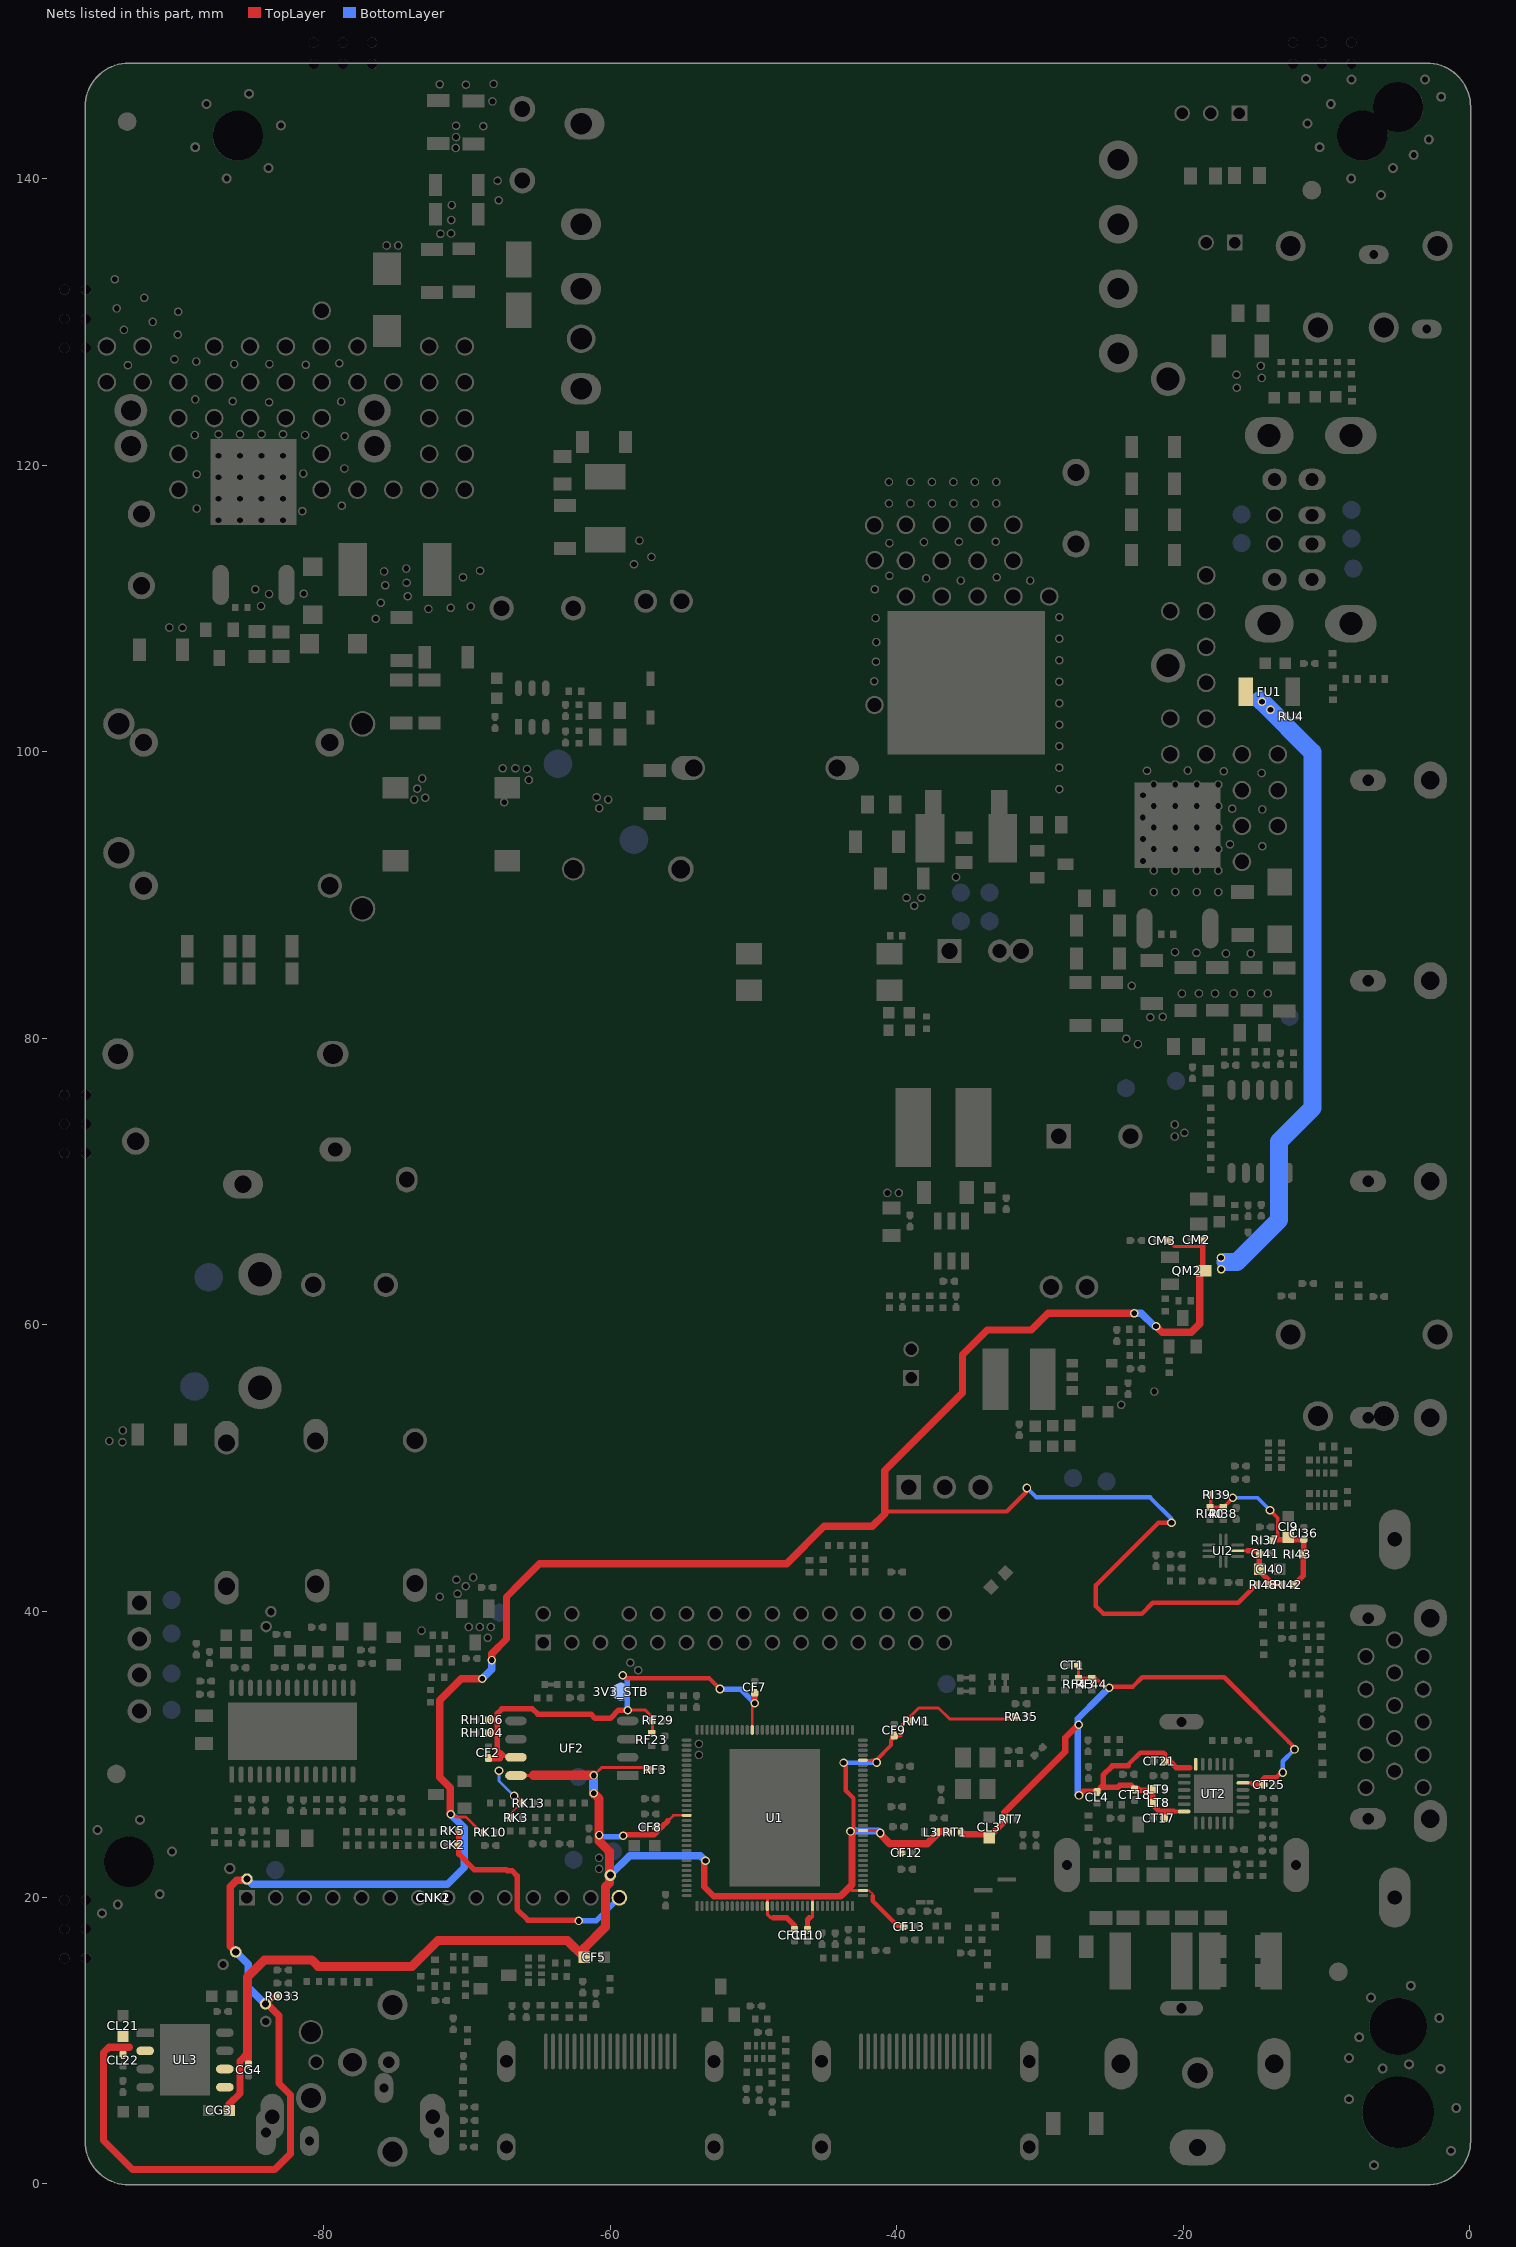
[diagram p0: the nets of this part, all layers, seen from the top]
# Altium PCB MISC86372.PcbDoc (part 6 of 16)
Units mm, origin at the board's own origin, x right, y up, seen from the top; angles counter-clockwise.
Board outline 96.73 x 148.13 mm, 2 copper layers (TopLayer, BottomLayer), stack 1.571 mm thick; 578 components, 318 nets, 2702 pads, 836 vias.

## Part data (continued)
RA36 RB804 RK15 RM12 RT7 RT8 RV6 RV8: library part 10Kohm-0402-±5%-1/16W-D
RB1 RB2 RB3 RB4: library part 1M2ohm-1206-±5%-1/4W-D, "RES"
RB101 RB102: library part 330Kohm-1206-±5%-1/4W-D, "RES"
RB103 RB109 RB808: library part 10Kohm-0402-±1%-1/16W-D
RB104: library part 47Kohm-0402-±1%-1/16W-D
RB105: library part 510ohm-0402-±1%-1/16W-D
RB106 RB113 RB121: library part 68ohm-0805-±5%-1/8W-D
RB107 RB807: library part 20ohm-0805-±5%-1/8W-D, "RES"
RB114: library part 4R7ohm-1206-±1%-1/4W-D, "RES"
RB117 RB118 RB119 RB120: library part 10ohm-1206-±5%-1/4W-D, "RES"
RB124 RB125 RB126 RB136: library part 68ohm-1206-±5%-1/4W-D
RB128 RB129: library part 47ohm-1206-±5%-1/4W-D, "RES"
RB130 RB143: library part 20ohm-1206-±5%-1/4W-D
RB131: library part 2Kohm-0603-±5%-1/10W-D
RB132 RB133 RB139: library part 3Kohm-0402-±1%-1/16W-D
RB134: library part 4K7ohm-0402-±1%-1/16W-D, "RES"
RB135: library part 18Kohm-0402-±1%-1/16W-D, "RES"
RB140: library part 51Kohm-0805-±1%-1/8W-D, "RES"
RB141 RB142: library part 2Mohm-1206-±5%-1/4W-D, "RES"
RB148: library part 厚膜电阻,RES,1W,0.24ohm,±1%,2512,SMD
RB150 RB151 RB152 RB153 RB825 RB826: library part 100Kohm-1206-±5%-1/4W-D, "RES"
RB803 RB813 RB833: library part 100ohm-0402-±5%-1/16W-D, "RES"
RB806 RK8: library part 1Kohm-0402-±1%-1/16W-D
RB814 RB816 RB834 RB835: library part 33ohm-0805-±5%-1/8W-D
RB818 RB819 RB820 RB821 RB822 RB823 RB824: library part 0R47ohm-1206-±1%-1/4W-D
RB845 RB846 RB847: library part 0ohm-0805-±5%-1/8W-D
RD3: library part 004.002.0000104-D, "Thick-film resistor,RES,1/16W,33Kohm,±1%,0402,SMD-D"
RD5: library part 004.002.0000717-D, "Thick-film resistor,RES,1/16W,6.04Kohm,±1%,0402,SMD-D"
RD6: library part 004.002.0000806-D, "Thick-film resistor,RES,1/16W,60.4Kohm,±1%,0402,SMD-D"
RD8: library part 004.002.0000593-D, "Thick-film resistor,RES,1/16W,13Kohm,±1%,0402,SMD-D"
RD9: library part 004.002.0000588-D, "Thick-film resistor,RES,1/16W,12Kohm,±1%,0402,SMD-D"
RF3 RF8 RF9 RF13 RF23 RF29 RF43 RF44 RK1 RM11 RM13 RM15: library part 4K7ohm-0402-±5%-1/16W-D
RF10 RF11 RI48 RV7 RV9: library part 100ohm-0402-±5%-1/16W-D
RF12 RF16 RH102 RH103 RH104 RH105 RH106: library part 68ohm-0402-±5%-1/16W-D
RFT1: library part "RF头,RF JACK,H,IEC,T14.5,CH6.3,12.4×13.2×7.7mm,DIP,LHD-020组件,LHD-DLMI", "T-IEC-6.3mm-#-#"
RFT2: library part "RF头,RF JACK,H,F,T14.5,CH6.3,without pipe,12.4×13.2×7.7mm,DIP,LHD-DLMI", "T-F-6.3mm-#-#"
RG61 RU1 RU2 RU3 RU5: library part 0ohm-0402-PCB-D, "0ohm-0402-PCB-D"
RH4 RH24 RPI1 RPV1 RPV2: library part 4*100ohm-0402-±5%-1/16W-D
RH5 RH6 RH25 RH26 RI2 RV2 RV4 RV10: library part 33ohm-0402-±5%-1/16W-D
RH81: library part 22Kohm-0402-±5%-1/16W-D
RH82 RK13: library part 33Kohm-0402-±5%-1/16W-D
RH83 RO22: library part 004.002.0000568-D, "Thick-film resistor,RES,1/16W,100ohm,±5%,0402,SMD-D"
RI1 RO1 RV1 RV3 RV5: library part 75ohm-0402-±5%-1/16W-D
RI5 RI6 RO4 RO33 RT4 RT5: library part 0ohm-0402-±5%-1/16W-D
RI37 RI38 RI39 RI40: library part 200Kohm-0402-±5%-1/16W-D
RK3 RK12: library part 4K7ohm-0402-±1%-1/16W-D
RK5 RT2 RT3: library part 22ohm-0402-±5%-1/16W-D
RK6 RK14 RO12 RO15: library part 510ohm-0402-±5%-1/16W-D
RK7: library part 680ohm-0402-±1%-1/16W-D
RK9: library part 1K2ohm-0402-±1%-1/16W-D
RK11: library part 2K2ohm-0402-±1%-1/16W-D
RK16: library part 15Kohm-0402-±1%-1/16W-D
RM1 RM2: library part 004.002.0000577-D, "Thick-film resistor,RES,1/16W,10Kohm,±5%,0402,SMD-D"
RT6: library part 1K8ohm-0402-±5%-1/16W-D
TB101: library part 004.004.0002645-DLMI, "Transformer,EQ2414,300uH,0.2×1P,26Ts,H14.5MAX,SYEQ2414Z-T012064B(BLACK),DIP,SQ-DLMI"
TP-TDT: library part TEST, "TEST"
U1: library part 004.016.0001146-D, "TV main chip,IC Main Chip,TSUMV53RWUT-Z1,32bit,Single-Core,QFN128,SMD,Mstar-D"
UA1: library part 004.012.0000190-D, "Audio amplifier,IC Audio AMP,Class D,2×10W@13.0V@8ohm,HTSSOP-28,SMD,RDA3118E28B,RDA-D"
UB101: library part 004.010.0000426, "PWM controller,IC PWM Controller,65KHZ,SOT23-6,SMD,OB2273C,ON-Bright-D"
UB801: library part SY7710FHC, "SSOP10"
UD1: library part 004.010.0000700-D, "DC-DC converter,IC DCDC,Syn,2A,18V,500KHz,SOT23-6,SMD,LC2332CB6TR,Leadchip-D"
UD2: library part "DC-DCоƬ,IC DCDC,Syn,1.2A,7.0V,1.5MHz,SOT23-5,SMD,LC2127CB5TR,Leadchip-D"
UF2: library part "SPI FLASH оƬ,IC SPI FLASH,32Mb,SOIC8,SMD,GD25Q32CSIG,GigaDevice-D"
UI2: library part AZAW2213F-D
UL3: library part 004.010.0000256-D, "LDO regulator,IC LDO,1A,3.3V,12V,ESOP-8,SMD,LC1118CS8TR1833,Leadchip-D"
UT2: library part "硅高频头,IC Si Tuner,QFN24,SMD,R842,Rafael-D"
YF1: library part 16.000MHz±20PPM-10PF-SMD3225-D
ZDB801: library part "TVS管,DIO ESD,400pF,24.4V,SMB,SMD,SMBJ15AHR4G,TSC-D", "TVS"
ZDB802: library part BZX84C24(蓝箭)-D, "Diode"
用于U1: library part Φ12mm×12mm-黑色-125度(UL认证)-D

## Free pads (board coordinates)
  round 0.7 hole 0.7 unplated: 0(-186.339,148) 0(-186.339,149.5) 0(-184.299,148) 0(-184.299,149.5) 0(-182.259,148) 0(-182.259,149.5) 0(-117.982,148) 0(-117.982,149.5) 0(-115.942,148) 0(-115.942,149.5) 0(-113.902,148) 0(-113.902,149.5) 0(-98.1,71.96) 0(-98.1,74) 0(-98.1,76.04) 0(-98.1,128.167) 0(-98.1,130.207) 0(-98.1,132.247) 0(-98.1,15.753) 0(-98.1,17.793) 0(-98.1,19.833) 0(-98.1,221.46) 0(-98.1,223.5) 0(-98.1,225.54) 0(-98.1,277.667) 0(-98.1,279.707) 0(-98.1,281.747) 0(-98.1,165.253) 0(-98.1,167.293) 0(-98.1,169.333) 0(-96.6,71.96) 0(-96.6,74) 0(-96.6,76.04) 0(-96.6,128.167) 0(-96.6,130.207) 0(-96.6,132.247) 0(-96.6,15.753) 0(-96.6,17.793) 0(-96.6,19.833) 0(-96.6,221.46) 0(-96.6,223.5) 0(-96.6,225.54) 0(-96.6,277.667) 0(-96.6,279.707) 0(-96.6,281.747) 0(-96.6,165.253) 0(-96.6,167.293) 0(-96.6,169.333) 0(-80.702,148) 0(-80.702,149.5) 0(-78.662,148) 0(-78.662,149.5) 0(-76.622,148) 0(-76.622,149.5) 0(-12.345,148) 0(-12.345,149.5) 0(-10.305,148) 0(-10.305,149.5) 0(-8.265,148) 0(-8.265,149.5)
  oval 4x5 on Keep-Out: 0(-5,125.3)
  rrect50% 20x15 on Keep-Out: 31(-46.939,135.585)
  round 4 on Keep-Out: 31(-33.528,143)
  round 1.3 hole 1 paste-0.65 mask-0.051: VIA5(-95.149,125.783) VIA5(-95.149,128.283) VIA5(-92.649,125.783) VIA5(-92.649,128.283) VIA5(-90.149,118.283) VIA5(-90.149,120.783) VIA5(-90.149,123.283) VIA5(-90.149,125.783) VIA5(-87.649,123.283) VIA5(-87.649,125.783) VIA5(-87.649,128.283) VIA5(-85.149,123.283) VIA5(-85.149,125.783) VIA5(-85.149,128.283) VIA5(-82.649,123.283) VIA5(-82.649,125.783) VIA5(-82.649,128.283) VIA5(-80.149,118.283) VIA5(-80.149,120.783) VIA5(-80.149,123.283) VIA5(-80.149,125.783) VIA5(-80.149,128.283) VIA5(-80.149,130.783) VIA5(-77.649,118.283) VIA5(-77.649,125.783) VIA5(-77.649,128.283) VIA5(-75.149,118.283) VIA5(-75.149,125.783) VIA5(-72.649,118.283) VIA5(-72.649,120.783) VIA5(-72.649,123.283) VIA5(-72.649,125.783) VIA5(-72.649,128.283) VIA5(-70.149,118.283) VIA5(-70.149,120.783) VIA5(-70.149,123.283) VIA5(-70.149,125.783) VIA5(-70.149,128.283) VIA5(-41.58,115.799) VIA5(-41.554,103.251) VIA5(-41.529,113.36) VIA5(-39.359,110.827) VIA5(-39.359,113.327) VIA5(-39.359,115.827) VIA5(-36.859,110.827) VIA5(-36.859,113.327) VIA5(-36.859,115.827) VIA5(-34.359,110.827) VIA5(-34.359,113.327) VIA5(-34.359,115.827) VIA5(-31.859,110.827) VIA5(-31.859,113.327) VIA5(-31.859,115.827) VIA5(-29.359,110.827) VIA5(-20.9,99.804) VIA5(-20.9,102.304) VIA5(-20.9,109.804) VIA5(-18.4,99.804) VIA5(-18.4,102.304) VIA5(-18.4,104.804) VIA5(-18.4,107.304) VIA5(-18.4,109.804) VIA5(-18.4,112.304) VIA5(-15.9,92.304) VIA5(-15.9,94.804) VIA5(-15.9,97.304) VIA5(-15.9,99.804) VIA5(-13.4,94.804) VIA5(-13.4,97.304) VIA5(-13.4,99.804)
  round 0.6 hole 0.4 paste-0.4 mask-0.4: VIA5(-94.971,51.867) VIA5(-94.59,132.969) VIA5(-94.463,130.937) VIA5(-94.056,51.791) VIA5(-94.031,52.603) VIA5(-93.955,129.438) VIA5(-93.675,126.975) VIA5(-92.532,131.674) VIA5(-91.948,129.997) VIA5(-90.78,108.661) VIA5(-90.424,127.381) VIA5(-90.195,129.108) VIA5(-90.17,130.708) VIA5(-89.865,108.636) VIA5(-89,122.098) VIA5(-88.976,124.587) VIA5(-88.9,127.229) VIA5(-88.875,116.967) VIA5(-88.875,119.355) VIA5(-87.348,116.156) VIA5(-87.348,117.656) VIA5(-87.348,119.156) VIA5(-87.348,120.656) VIA5(-87.348,122.156) VIA5(-86.36,124.46) VIA5(-86.258,127.051) VIA5(-85.848,116.156) VIA5(-85.848,117.656) VIA5(-85.848,119.156) VIA5(-85.848,120.656) VIA5(-85.848,122.156) VIA5(-84.785,111.328) VIA5(-84.379,110.16) VIA5(-84.348,116.156) VIA5(-84.348,117.656) VIA5(-84.348,119.156) VIA5(-84.348,120.656) VIA5(-84.348,122.156) VIA5(-83.82,110.998) VIA5(-83.82,124.384) VIA5(-83.795,127.051) VIA5(-82.848,116.156) VIA5(-82.848,117.656) VIA5(-82.848,119.156) VIA5(-82.848,120.656) VIA5(-82.848,122.156) VIA5(-81.501,116.783) VIA5(-81.432,119.405) VIA5(-81.407,111.023) VIA5(-81.305,122.098) VIA5(-81.255,127) VIA5(-78.918,127.102) VIA5(-78.791,124.435) VIA5(-78.74,117.17) VIA5(-78.562,119.761) VIA5(-78.537,122.022) VIA5(-76.378,109.271) VIA5(-76.022,110.388) VIA5(-75.794,112.573) VIA5(-75.717,111.608) VIA5(-75.616,135.331) VIA5(-74.803,135.331) VIA5(-74.244,112.776) VIA5(-74.219,111.785) VIA5(-74.143,110.846) VIA5(-73.685,96.647) VIA5(-73.482,97.409) VIA5(-73.177,38.633) VIA5(-73.127,98.12) VIA5(-72.923,96.774) VIA5(-72.695,109.957) VIA5(-71.907,40.996) VIA5(-71.907,146.583) VIA5(-71.857,136.144) VIA5(-71.145,110.033) VIA5(-71.12,136.169) VIA5(-71.095,137.109) VIA5(-71.065,138.151) VIA5(-70.79,142.138) VIA5(-70.764,142.9) VIA5(-70.764,143.688) VIA5(-70.739,42.189) VIA5(-70.663,41.199) VIA5(-70.282,112.166) VIA5(-70.098,41.732) VIA5(-70.079,146.558) VIA5(-69.875,38.887) VIA5(-69.748,110.134) VIA5(-69.571,42.342) VIA5(-69.108,38.887) VIA5(-69.088,112.624) VIA5(-68.859,143.662) VIA5(-68.555,38.125) VIA5(-68.34,38.887) VIA5(-68.224,145.39) VIA5(-68.148,146.609) VIA5(-67.869,139.852) VIA5(-67.793,138.481) VIA5(-67.513,98.831) VIA5(-67.412,96.469) VIA5(-66.624,98.831) VIA5(-65.811,98.781) VIA5(-65.684,98.019) VIA5(-60.955,96.809) VIA5(-60.782,21.996) VIA5(-60.782,22.764) VIA5(-60.776,96.054) VIA5(-60.147,96.647) VIA5(-58.602,36.394) VIA5(-58.344,113.081) VIA5(-58.054,35.871) VIA5(-57.963,114.732) VIA5(-57.125,113.589) VIA5(-53.811,29.954) VIA5(-53.811,30.722) VIA5(-41.58,104.902) VIA5(-41.529,111.328) VIA5(-41.478,109.322) VIA5(-41.453,106.274) VIA5(-41.427,107.645) VIA5(-40.654,69.19) VIA5(-40.545,117.321) VIA5(-40.545,118.821) VIA5(-40.513,112.268) VIA5(-40.513,114.554) VIA5(-39.853,69.19) VIA5(-39.319,89.789) VIA5(-39.045,117.321) VIA5(-39.045,118.821) VIA5(-38.786,89.23) VIA5(-38.278,89.789) VIA5(-38.1,114.63) VIA5(-37.948,112.09) VIA5(-37.545,118.821) VIA5(-37.545,117.321) VIA5(-36.045,117.321) VIA5(-36.045,118.821) VIA5(-35.865,91.237) VIA5(-35.662,114.656) VIA5(-35.535,111.938) VIA5(-34.545,117.321) VIA5(-34.545,118.821) VIA5(-33.096,114.656) VIA5(-33.045,117.321) VIA5(-33.045,118.821) VIA5(-33.02,112.166) VIA5(-30.683,111.938) VIA5(-28.651,97.378) VIA5(-28.651,98.878) VIA5(-28.651,100.378) VIA5(-28.651,101.878) VIA5(-28.651,103.378) VIA5(-28.651,104.878) VIA5(-28.651,106.378) VIA5(-28.651,107.878) VIA5(-28.651,109.378) VIA5(-24.337,54.392) VIA5(-23.978,79.959) VIA5(-23.597,83.642) VIA5(-23.422,60.782) VIA5(-23.165,79.578) VIA5(-22.835,95.402) VIA5(-22.809,92.354) VIA5(-22.809,93.904) VIA5(-22.809,96.952) VIA5(-22.53,98.654) VIA5(-22.301,81.458) VIA5(-22.051,90.195) VIA5(-22.051,91.695) VIA5(-22.051,93.195) VIA5(-22.051,94.695) VIA5(-22.051,96.195) VIA5(-22.051,97.695) VIA5(-22.022,55.321) VIA5(-21.438,81.483) VIA5(-20.599,73.127) VIA5(-20.599,73.965) VIA5(-20.574,86.004) VIA5(-20.551,90.195) VIA5(-20.551,91.695) VIA5(-20.551,93.195) VIA5(-20.551,94.695) VIA5(-20.551,96.195) VIA5(-20.551,97.695) VIA5(-20.091,83.109) VIA5(-19.914,73.381) VIA5(-19.685,98.679) VIA5(-19.075,85.954) VIA5(-19.051,90.195) VIA5(-19.051,91.695) VIA5(-19.051,93.195) VIA5(-19.051,94.695) VIA5(-19.051,96.195) VIA5(-19.051,97.695) VIA5(-18.907,83.114) VIA5(-17.78,83.114) VIA5(-17.551,90.195) VIA5(-17.551,91.695) VIA5(-17.551,93.195) VIA5(-17.551,94.695) VIA5(-17.551,96.195) VIA5(-17.551,97.695) VIA5(-17.366,64.665) VIA5(-17.348,63.856) VIA5(-17.17,98.628) VIA5(-17.018,85.903) VIA5(-16.739,93.523) VIA5(-16.586,96.012) VIA5(-16.485,83.114) VIA5(-16.281,126.314) VIA5(-16.256,125.4) VIA5(-15.291,85.903) VIA5(-15.265,83.114) VIA5(-14.58,126.924) VIA5(-14.529,98.501) VIA5(-14.527,126.087) VIA5(-14.503,103.48) VIA5(-14.478,93.396) VIA5(-14.478,95.961) VIA5(-14.097,83.114) VIA5(-13.911,102.914)
  round 0.8 hole 0.5 paste-0.4 mask-0.4: VIA5(-87.027,15.327) VIA5(-86.563,22.022) VIA5(-86.148,16.205) VIA5(-85.365,21.29) VIA5(-84.074,12.573) VIA5(-84.051,11.354) VIA5(-84.023,38.913) VIA5(-83.693,39.954)

## Via types
v1: diameter 0.6, hole 0.4, TopLayer to BottomLayer, tented both sides, 816 vias
v2: diameter 0.7, hole 0.5, TopLayer to BottomLayer, tented both sides, 15 vias
v3: diameter 0.8, hole 0.5, TopLayer to BottomLayer, tented both sides, 5 vias

## Nets (pads, with @x,y where several pads share a name; then routed paths per layer and width w, separated by ;. In a path a pad name is that pad's centre, name@x,y a point inside that pad or via, vN(x,y) a via of type N, cw(c..) or ccw(c..) an arc to the next point about the centre after c; other vN are vias at no path point)
2V5_ASW: CI9.2 CI36.2@-11.582,44.99 CI36.2@-11.582,45.165 RI37.2 RI38.2 RI39.2 RI40.2 RI42.2 RI43.2 | length 13.6
  TopLayer w0.254: RI39.2@-18.078,48.133 -18.078,47.278 RI40.2@-18.127,47.23 RI38.2@-17.213,47.23 v1@-16.551,47.891 ; v1(-13.945,47.041) -13.396,46.492 -13.396,45.166
  TopLayer w0.381: RI37.2@-13.85,44.929 -13.788,44.99 CI36.2@-11.582,44.99 -11.582,44 RI43.2@-11.615,43.967 -11.615,42.469 RI42.2@-12.25,41.834
  BottomLayer w0.254: v1(-16.551,47.907) -14.811,47.907 v1(-13.945,47.041)
3V3_STB: 3V3_STB.1 CF2.2@-68.504,29.69 CF2.2@-68.504,29.865 CF5.2 CF7.2@-49.911,34.246 CF7.2@-49.911,34.421 CF8.2@-56.777,24.914 CF8.2@-56.952,24.914 CF9.2@-40.174,31.264 CF9.2@-40.174,31.439 CF10.2@-46.226,17.8 CF10.2@-46.226,17.625 CF11.1 CF12.2@-39.544,23.114 CF12.2@-39.719,23.114 CF13.2@-39.54,17.975 CF13.2@-39.365,17.975 CG3.2 CG4.1 L3.1 RA35.2 RF3.2 RF23.2 RF29.2 RH104.2 RH106.2 RK3.2 RK13.2 RM1.2 RT1.2 U1.15 U1.24 U1.34 U1.46 U1.60 U1.85 U1.112 UF2.7 UF2.8 UL3.5 UL3.6 | length 173.3
  TopLayer w0.127: RK3.2@-67,25.569 -67,25.823 RK13.2@-66.229,26.594 ; U1.34@-42.363,20.481 -41.918,20.481 -41.685,20.248 -41.685,20.107
  TopLayer w0.178: -55.978,25.345 -55.592,25.731 U1.112@-54.663,25.731 ; U1.85@-50.088,31.707 U1.85@-50.088,31.707 CF7.2@-50.088,34.455
  TopLayer w0.203: v1(-66.718,27.094) -66.604,27.094 RK13.2@-66.104,26.594 RK13.2@-66.091,26.594 ; UF2.8@-66.587,28.515 -65.389,28.515 ; v1(-61.163,28.524) -60.602,29.085 -57.445,29.085 RF3.2@-57.29,28.931 RF3.2@-57.364,28.857 ; v1(-58.783,33.077) -57.546,33.077 -57.048,32.579 RF23.2@-57.048,31.556 ; -49.038,20.05 U1.15@-49.038,19.406 -49.038,18.827 -48.794,18.582 ; -46.231,18.3 -45.888,18.643 U1.24@-45.888,19.406 -45.888,20.086 -45.888,20.138 ; -43.337,20.676 -43.141,20.481 U1.34@-42.363,20.481 ; v1@-43.091,24.681 U1.46@-42.413,24.681 ; U1.46@-42.362,24.681 -41.358,24.681 v1@-41.121,24.443 ; U1.60@-42.362,29.581 -41.736,29.581 ; -41.717,29.562 -41.736,29.581 ; v1(-41.411,29.427) -41.546,29.562 -41.564,29.581 -41.736,29.581 ; CF9.2@-40.278,31.115 CF9.2@-40.278,31.257 ; CF9.2@-40.174,31.264 -39.755,31.264 -39.599,31.42 -39.599,32.095 -38.458,33.235 -37.083,33.235 -36.321,32.474 -31.883,32.474 RA35.2@-31.743,32.614
  TopLayer w0.279: -41.717,29.562 -41.546,29.562 -41.458,29.562 -40.391,30.629 -40.391,31.002 CF9.2@-40.278,31.115
  TopLayer w0.305: v1(-59.131,35.509) -58.931,35.309 -53.097,35.309 ; -53.081,35.293 v1(-52.342,34.554) ; v1@-43.778,29.401 -43.551,29.174 -43.551,27.459 -43.017,26.925 -43.017,24.826 v1(-43.231,24.613) ; -41.685,20.107 -41.685,19.767 -39.893,17.975 CF13.2@-39.54,17.975
  TopLayer w0.381: RH104.2@-68.511,31.487 -67.909,31.487 ; RH106.2@-68.511,32.401 -67.883,32.401 ; CF2.2@-68.504,29.69 -67.672,29.69 ; -67.883,29.749 -67.883,32.401 ; -67.672,30.122 -67.488,29.937 ; v1@-59.194,24.372 v1@-59.042,24.372 ; v1@-59.08,24.333 v1@-59.042,24.372 ; v1@-58.946,24.372 -57.534,24.372 ; v1(-58.783,33.077) -59.425,33.077 -59.991,32.512 -61.05,32.512 -61.332,32.795 -65.051,32.795 -65.429,33.172 -67.569,33.172 -67.883,32.858 -67.883,32.401 ; CF8.2@-56.777,24.94 -56.383,24.94 ; -55.978,25.345 -56.383,24.94 ; v1@-52.342,34.655 v1(-52.342,34.554) v1@-52.332,34.544 ; v1(-49.911,33.553) CF7.2@-49.911,34.246 ; -48.61,18.582 -47.665,18.582 -47.145,18.062 ; CF10.2@-46.226,17.625 -46.231,17.63 -46.231,18.3 -46.231,18.462 -46.105,18.588 ; -39.751,23.759 -39.719,23.727 CF12.2@-39.719,23.114 ; v1@-59.042,24.372 -57.534,24.372 ; -57.534,24.372 -56.95,24.372 -56.383,24.94
  TopLayer w0.432: v1(-53.354,22.566) -53.438,22.482 -53.438,20.751 -52.773,20.086 -45.888,20.086 -43.927,20.086 -43.826,20.187
  TopLayer w0.508: CG3.2@-86.616,5.13 -86.616,5.56 -85.855,6.321 -85.855,8.589 -85.325,9.119 ; -43.826,20.187 -43.337,20.676 -43.119,20.894 -43.119,24.501 v1(-43.231,24.613) ; v1@-41.121,24.443 -41.121,24.397 -40.483,23.759 -39.751,23.759 -37.869,23.759 -37.218,24.41 L3.1@-37.218,24.563 ; L3.1@-37.218,24.424 -37.218,24.613 -37.215,24.615 RT1.2@-36.366,24.615
  TopLayer w0.635: -85.325,8.747 -85.325,9.119 -85.325,14.457 -84.136,15.646 -80.85,15.646 -80.392,15.189 -73.841,15.189 -72.037,16.993 -62.987,16.993 CF5.2@-61.819,15.824 -61.819,16.464 -60.334,17.949 -60.334,20.743 -60.048,21.029 -60.048,23.208 -60.774,23.934 v1(-60.774,24.359) -60.774,26.881 v1(-61.163,27.27) ; -65.372,28.532 v1@-61.163,28.532
  BottomLayer w0.203: v1(-67.767,28.854) -67.767,28.143 v1(-66.718,27.094)
  BottomLayer w0.305: v1@-43.79,29.413 v1@-43.786,29.409 ; v1@-43.778,29.401 v1@-43.786,29.409 ; v1(-43.713,29.413) v1@-43.709,29.409 ; v1@-41.554,29.409 v1@-43.709,29.409 ; v1@-43.786,29.409 v1@-43.709,29.409
  BottomLayer w0.381: v1@-60.774,24.257 -59.36,24.257 -59.131,24.257 v1(-59.085,24.303) ; v1(-59.131,35.509) -58.809,35.187 v1@-58.809,33.077 ; v1(-52.342,34.554) -50.911,34.554 v1(-49.911,33.553)
  BottomLayer w0.508: v3@-59.969,21.539 v3(-59.995,21.565) -58.637,22.922 -53.71,22.922 v1(-53.354,22.566) ; v1@-43.231,24.638 -41.297,24.638 v1(-41.161,24.502)
  BottomLayer w0.635: v1(-61.163,27.27) v1(-61.163,28.524)
3V3_TUNER: CL3.2 CL4.2@-26.01,27.238 CL4.2@-26.01,27.413 CT1.1 CT17.2@-21.292,25.532 CT17.2@-21.467,25.532 CT18.1 CT21.2@-21.241,29.515 CT21.2@-21.416,29.515 CT25.1 LT8.1 LT9.2 RF43.1 RF44.1 RT1.1 RT7.1 UT2.11 UT2.18 UT2.24 | length 63.7
  TopLayer w0.203: RF43.1@-27.312,35.332 CT1.1@-27.312,36.22 ; RF43.1@-27.305,35.325 -26.1,35.325 -25.795,35.02 -25.421,34.646 v1(-25.171,34.646)
  TopLayer w0.249: -20.65,26.006 -20.648,26.004 UT2.24@-19.932,26.004 ; UT2.11@-15.832,28.004 -15.203,28.004
  TopLayer w0.305: v1(-25.171,34.646) -25.095,34.722 -24.054,34.722 ; -24.562,34.722 -24.054,34.722 ; -23.8,29.319 -23.008,30.11 -21.372,30.11 -21.26,29.997 -21.26,29.717 CT21.2@-21.241,29.698 ; CT25.1@-14.446,27.864 -14.446,28.273 -14.326,28.393 ; -14.021,28.393 -14.326,28.393 ; v1(-13.056,28.727) -13.146,28.727 -13.48,28.393 -14.326,28.393 ; -12.374,30.603 -12.653,30.882 ; v1(-12.23,30.338) -12.23,30.459 -12.653,30.882 ; -24.054,34.722 -23.512,34.722 -22.864,35.369 -17.14,35.369 -12.653,30.882
  TopLayer w0.381: v1(-27.28,27.127) -26.993,27.413 CL4.2@-26.01,27.413 ; -23.851,29.185 -24.945,29.185 -25.586,28.544 -25.586,27.837 CL4.2@-26.01,27.413 ; CT18.1@-23.393,27.603 -23.611,27.821 -24.437,27.821 -24.55,27.707 -25.716,27.707 CL4.2@-26.01,27.413 ; CT18.1@-23.17,27.605 -23.04,27.475 -22.231,27.475 LT9.2@-22.142,27.564 LT8.1@-22.142,26.599 -22.142,26.5 -21.648,26.006 ; -21.628,26.015 ccw(c-21.628,25.987) -21.648,26.006 ; -21.292,25.906 CT17.2@-21.292,25.532 CT17.2@-21.26,25.564 ; CT21.2@-21.241,29.515 -20.93,29.515 -20.472,29.058 -19.558,29.058 ; -20.65,26.006 -21.648,26.006 ; -15.113,27.915 CT25.1@-14.471,27.915 ; CT25.1@-14.471,27.889 CT25.1@-14.446,27.864
  TopLayer w0.457: RT1.1@-35.516,24.566 -35.355,24.405 -33.772,24.405 CL3.2@-33.55,24.182 ; CL3.2@-33.535,24.391 -33.477,24.333 -32.48,25.331 -32.48,25.951 -28.245,30.186 -28.245,31.146 -27.326,32.064 v1(-27.289,32.064)
  BottomLayer w0.305: v1(-13.056,28.727) -13.056,29.513 v1(-12.23,30.338)
  BottomLayer w0.457: v1(-27.28,27.127) -27.361,27.208 -27.361,32.482 -25.768,34.074 v1@-25.324,34.519
5V_ASW: CI40.2 CI41.2@-14.7,43.993 CI41.2@-14.525,43.993 RI42.1 RI48.2 UI2.9 | length 4.9
  TopLayer w0.178: UI2.9@-16.206,44.208 -15.506,44.208 -15.494,44.196
  TopLayer w0.305: RI48.2@-13.977,41.834 RI42.1@-13.1,41.834
  TopLayer w0.381: -15.494,44.196 -14.903,44.196 CI41.2@-14.7,43.993 -14.681,43.974 -14.681,42.799 -13.977,42.095 RI48.2@-13.977,41.834
5V_IR: CK2.2@-70.75,23.688 CK2.2@-70.575,23.688 CNK1.14 CNK2.14 RK5.2 | length 16.8
  TopLayer w0.381: CK2.2@-70.575,23.688 -70.575,23.026 -69.482,21.933 -67.267,21.933 -67.192,21.858 -66.841,21.858 -66.497,21.514 -66.497,19.63 -66.497,19.163 -65.757,18.422 -62.261,18.422 v1(-62.205,18.365) ; CK2.2@-70.568,23.688 RK5.2@-70.568,24.669
  BottomLayer w0.381: v1(-62.205,18.365) -60.989,18.365 CNK2.14@-59.365,19.99
5V_M: CL21.1 CL22.1 CM2.2@-18.628,65.913 CM2.2@-18.803,65.913 CM3.1 FU1.2 pad.VIA5@-13.911,102.914 pad.VIA5@-14.503,103.48 pad.VIA5@-17.348,63.856 pad.VIA5@-17.366,64.665 pad.VIA5@-23.422,60.782 pad.VIA5@-84.074,12.573 pad.VIA5@-85.365,21.29 pad.VIA5@-86.148,16.205 QM2.D RI48.1 RK10.2 RO33.1 RU4.2 UL3.2 | length 242.9
  TopLayer w0.203: v1@-71.056,25.886 -70.782,25.611 -70.071,25.611 -69.004,24.544 RK10.2@-68.82,24.544 ; CM3.1@-21.028,65.862 -20.625,65.46 -18.657,65.46 -18.628,65.43
  TopLayer w0.305: pad.VIA5@-84.074,12.573 -83.966,12.573 -83.432,13.106 RO33.1@-83.28,13.106 ; -40.843,46.949 -32.318,46.949 -30.912,48.355 v1(-30.912,48.59) ; -26.081,41.818 -26.098,41.8 ; v1(-20.819,46.165) -21.734,46.165 -26.098,41.8 ; RI48.1@-14.827,41.834 -14.907,41.834 -16.165,40.576 -22.127,40.576 -22.888,39.816 -25.576,39.816 -26.098,40.338 -26.098,41.8
  TopLayer w0.381: CM2.2@-18.628,65.913 -18.628,65.43 -18.628,63.813 QM2.D@-18.576,63.762
  TopLayer w0.508: -93.586,9.55 -95.001,9.55 -95.377,9.175 -95.377,3.03 -93.362,1.015 -93.244,1.015 -93.232,1.003 -83.44,1.003 -82.331,2.112 -82.331,6.213 -83.134,7.016 -83.134,11.742 pad.VIA5@-83.966,12.573 ; pad.VIA5@-86.148,16.205 -86.525,16.582 -86.525,20.755 -86.072,21.209 -85.445,21.209 pad.VIA5@-85.365,21.29 ; -71.907,28.857 -71.907,29.235 ; v1(-71.133,25.81) -71.179,25.856 -71.179,27.671 -71.907,28.399 -71.907,29.235 ; v1(-68.936,35.266) -70.413,35.266 -71.907,33.772 -71.907,29.235 ; v1(-68.275,36.576) -68.275,37.022 -67.247,38.05 -67.247,40.985 -66.228,42.003 -64.934,43.298 -47.689,43.298 -45.073,45.914 -41.702,45.914 -40.843,46.772 -40.843,46.949 -40.843,48.133 ; -40.843,47.566 -40.843,48.133 ; pad.VIA5@-23.422,60.782 -29.442,60.782 -30.611,59.614 -33.682,59.614 -35.408,57.888 -35.408,55.244 -40.843,49.809 -40.843,48.133 ; v1(-21.895,59.872) -21.484,59.461 -19.431,59.461 -18.841,60.051 -18.841,63.497 QM2.D@-18.576,63.762
  BottomLayer w0.305: v1(-30.912,48.59) -30.251,47.93 -22.311,47.93 -20.819,46.438 v1(-20.819,46.165)
  BottomLayer w0.508: pad.VIA5@-86.148,16.205 -85.281,15.337 -85.281,13.735 -84.118,12.573 pad.VIA5@-84.074,12.573 ; pad.VIA5@-85.365,21.29 -84.992,20.917 -71.364,20.917 -70.193,22.088 -70.193,24.87 v1(-71.133,25.81) ; v1(-68.936,35.266) -68.275,35.927 v1(-68.275,36.576) ; pad.VIA5@-23.422,60.782 -22.924,60.782 v1@-22.014,59.872
  BottomLayer w1.27: -17.043,64.364 -16.256,64.364 -13.31,67.31 -13.31,72.775 -10.973,75.112 -10.973,99.949 pad.VIA5@-14.503,103.48 pad.VIA5@-14.622,103.598